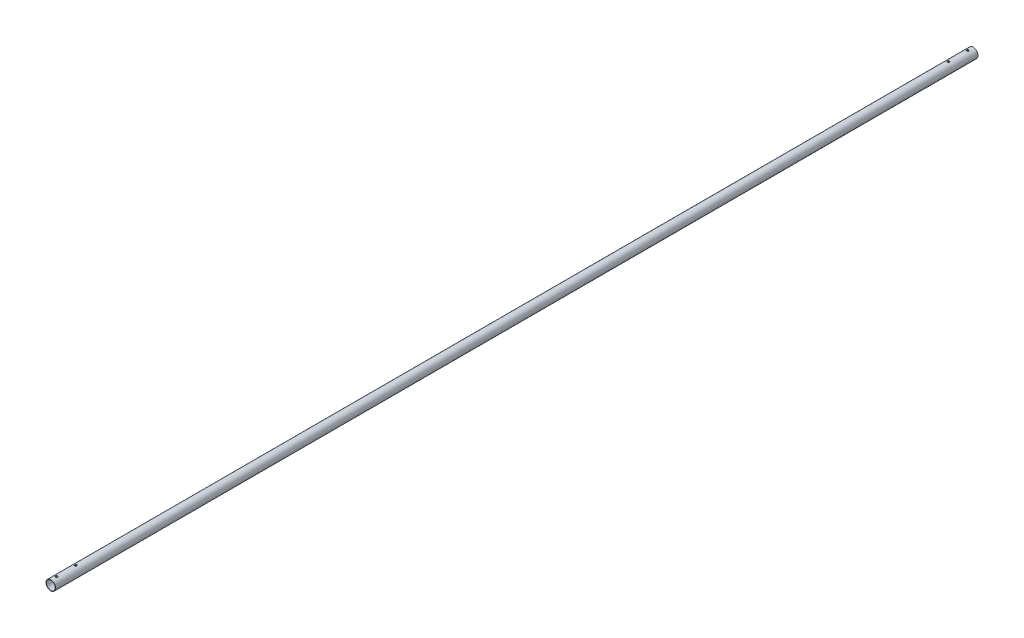
SolidWorks part; units mm, degrees
material "Thornel Mat VMA"
ref_plane "前视基准面" through (0, 0, 0) normal (0, 0, 1) x (1, 0, 0)
ref_plane "上视基准面" through (0, 0, 0) normal (0, 1, 0) x (1, 0, 0)
ref_plane "右视基准面" through (0, 0, 0) normal (1, 0, 0) x (0, 0, -1)
other "Configuration Table"
sketch "草图2" plane through (0, 0, 0) normal (0, 0, 1) x (1, 0, 0)
  circle A0 centre (0, 0) radius 7
  circle A1 centre (0, 0) radius 6.5
  dimension "D1" = 14
  dimension "D2" = 0.5
extrude "凸台-拉伸2" add sketch "草图2" along normal blind 1336
sketch "草图3" plane through (0, 0, 0) normal (0, 1, 0) x (1, 0, 0)
  line L0 (0, 0) -> (0, -90.2927) construction
  line L1 (7, 0) -> (-7, 0) construction
  line L2 (-7, -1336) -> (7, -1336) construction
  circle A0 centre (0, -8) radius 1.55
  circle A1 centre (0, -36) radius 1.55
  circle A2 centre (0, -1328) radius 1.55
  circle A3 centre (0, -1300) radius 1.55
  dimension "D1" = 3.1
  dimension "D2" = 8
  dimension "D3" = 28
  dimension "D4" = 8
  dimension "D5" = 28
extrude "切除-拉伸1" cut sketch "草图3" against normal through all both and the other way through all
